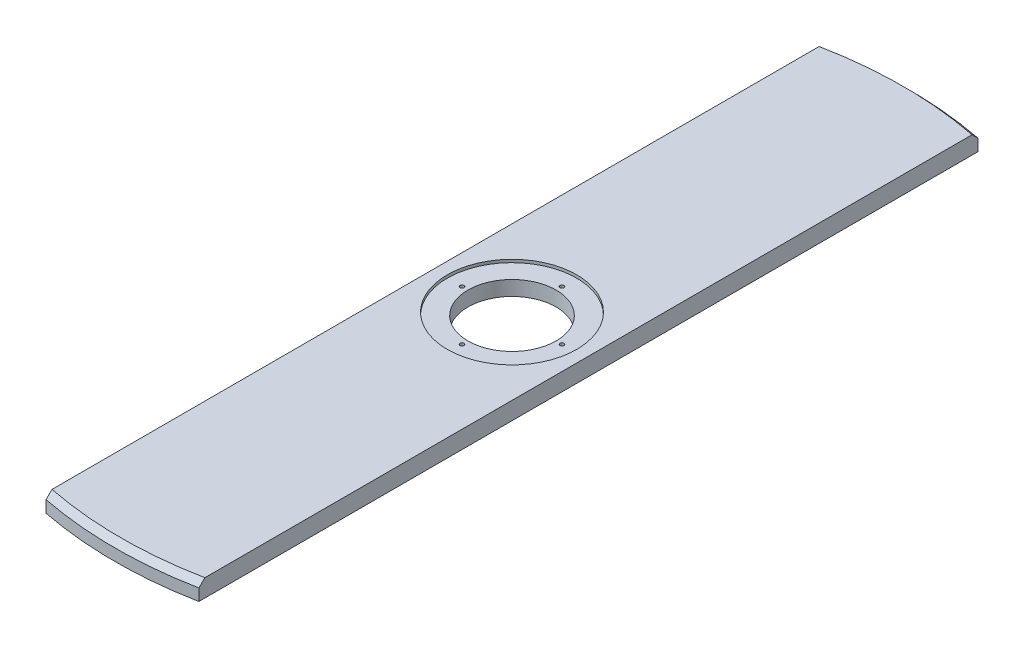
from build123d import *

# Parameters (mm, degrees)
SKETCH_1_R                = 810
EXTRUDE_1_DEPTH           = 25
SKETCH_2_R                = 730
EXTRUDE_2_DEPTH           = 5
CUT_EXTRUDE_1_REACH       = 1147.906
SKETCH_3_R                = 75
SKETCH_4_R                = 110
CUT_EXTRUDE_2_DEPTH       = 5
HOLE_WIZARD_M8_1_D        = 6.8
HOLE_WIZARD_25_5_25_5_1_D = 26
CUT_EXTRUDE_3_DEPTH       = 1146.905755287
CUT_EXTRUDE_3_DEPTH_BACK  = 1146.905755287
SKETCH_10_OUTSIDE_W       = 2080.244
SKETCH_10_OUTSIDE_H       = 2080.244
SKETCH_10_OUTSIDE_R       = 675
CHAMFER_1_SIZE            = 10


with BuildPart() as part:
    # 草图1 → 凸台-拉伸1 (new body)
    with BuildSketch(Plane(origin=(0, 0, 0), x_dir=(1, 0, 0), z_dir=(0, 1, 0))):
        with Locations(Location((0, 0, 0), (0, 0, 270))):
            Circle(SKETCH_1_R)
    extrude(amount=EXTRUDE_1_DEPTH)

    # 草图2 → 凸台-拉伸2 (add)
    with BuildSketch(Plane(origin=(0, 25, 0), x_dir=(1, 0, 0), z_dir=(0, 1, 0))):
        with Locations(Location((0, 0, 0), (0, 0, 270))):
            Circle(SKETCH_2_R)
    extrude(amount=EXTRUDE_2_DEPTH)

    # 草图3 → 切除-拉伸1 (cut, up to next)
    with BuildSketch(Plane(origin=(0, 30, 0), x_dir=(1, 0, 0), z_dir=(0, 1, 0)), mode=Mode.PRIVATE) as cut_extrude_1_sk1:
        with BuildLine():
            Line((130, 662.363193422), (130, -662.363193422))
            ThreePointArc((130, -662.363193422), (521.236510617, -428.879353665), (675, 0))
            ThreePointArc((675, 0), (521.236510617, 428.879353665), (130, 662.363193422))
        make_face()
    cut_extrude_1_tool1 = extrude(cut_extrude_1_sk1.sketch, amount=-CUT_EXTRUDE_1_REACH, mode=Mode.PRIVATE) & part.part
    # 草图3 → 切除-拉伸1 (cut, up to next)
    with BuildSketch(Plane(origin=(0, 30, 0), x_dir=(1, 0, 0), z_dir=(0, 1, 0)), mode=Mode.PRIVATE) as cut_extrude_1_sk2:
        with BuildLine():
            ThreePointArc((-130, 662.363193422), (-675, 0), (-130, -662.363193422))
            Line((-130, -662.363193422), (-130, 662.363193422))
        make_face()
    cut_extrude_1_tool2 = extrude(cut_extrude_1_sk2.sketch, amount=-CUT_EXTRUDE_1_REACH, mode=Mode.PRIVATE) & part.part
    # 草图3 → 切除-拉伸1 (cut, up to next)
    with BuildSketch(Plane(origin=(0, 30, 0), x_dir=(1, 0, 0), z_dir=(0, 1, 0)), mode=Mode.PRIVATE) as cut_extrude_1_sk3:
        with Locations(Location((0, 0, 0), (0, 0, 270))):
            Circle(SKETCH_3_R)
    cut_extrude_1_tool3 = extrude(cut_extrude_1_sk3.sketch, amount=-CUT_EXTRUDE_1_REACH, mode=Mode.PRIVATE) & part.part
    add(cut_extrude_1_tool1.solids().sort_by_distance((357.907844, 30, 0))[0], mode=Mode.SUBTRACT)
    add(cut_extrude_1_tool2.solids().sort_by_distance((-357.907844, 30, 0))[0], mode=Mode.SUBTRACT)
    add(cut_extrude_1_tool3.solids().sort_by_distance((0, 30, 0))[0], mode=Mode.SUBTRACT)

    # 草图4 → 切除-拉伸2 (cut)
    with BuildSketch(Plane(origin=(0, 30, 0), x_dir=(1, 0, 0), z_dir=(0, 1, 0))):
        with Locations(Location((0, 0, 0), (0, 0, 270))):
            Circle(SKETCH_4_R)
    extrude(amount=-CUT_EXTRUDE_2_DEPTH, mode=Mode.SUBTRACT)

    # M8 螺纹孔1 (through all)
    with Locations(Plane(origin=(0, 25, 0), x_dir=(1, 0, 0), z_dir=(0, 1, 0))):
        with Locations((0, 85), (85, 0), (0, -85), (-85, 0)):
            Hole(HOLE_WIZARD_M8_1_D / 2)

    # Ø25.5 (25.5) 直径孔1 (through all)
    with Locations(Plane(origin=(0, 25, 0), x_dir=(1, 0, 0), z_dir=(0, 1, 0))):
        with Locations((-59.354305918, 754.167962969), (59.354305918, 754.167962969), (176.601417757, 735.597844781), (289.500016584, 698.914866345), (395.270164208, 645.022284334), (491.307448562, 575.247112976), (575.247112976, 491.307448562), (645.022284334, 395.270164208), (698.914866345, 289.500016584), (735.597844781, 176.601417757), (754.167962969, 59.354305918), (754.167962969, -59.354305918), (735.597844781, -176.601417757), (698.914866345, -289.500016584), (645.022284334, -395.270164208), (575.247112976, -491.307448562), (491.307448562, -575.247112976), (395.270164208, -645.022284334), (289.500016584, -698.914866345), (176.601417757, -735.597844781), (59.354305918, -754.167962969), (-59.354305918, -754.167962969), (-176.601417757, -735.597844781), (-289.500016584, -698.914866345), (-395.270164208, -645.022284334), (-491.307448562, -575.247112976), (-575.247112976, -491.307448562), (-645.022284334, -395.270164208), (-698.914866345, -289.500016584), (-735.597844781, -176.601417757), (-754.167962969, -59.354305918), (-754.167962969, 59.354305918), (-735.597844781, 176.601417757), (-698.914866345, 289.500016584), (-645.022284334, 395.270164208), (-575.247112976, 491.307448562), (-491.307448562, 575.247112976), (-395.270164208, 645.022284334), (-289.500016584, 698.914866345), (-176.601417757, 735.597844781)):
            Hole(HOLE_WIZARD_25_5_25_5_1_D / 2)

    # 草图10 outside → 切除-拉伸3 (cut, two sides: drawn at the far end of the back side and taken through both)
    with BuildSketch(Plane(origin=(0, 30, 0), x_dir=(1, 0, 0), z_dir=(0, 1, 0)).offset(-CUT_EXTRUDE_3_DEPTH_BACK)):
        Rectangle(SKETCH_10_OUTSIDE_W, SKETCH_10_OUTSIDE_H)
        Circle(SKETCH_10_OUTSIDE_R, mode=Mode.SUBTRACT)
    extrude(amount=CUT_EXTRUDE_3_DEPTH + CUT_EXTRUDE_3_DEPTH_BACK, mode=Mode.SUBTRACT)

    # 倒角1
    chamfer_1_edges = [part.edges().sort_by_distance(p)[0] for p in [
        (0, 30, -675),
        (0, 30, 675),
    ]]
    chamfer(chamfer_1_edges, length=CHAMFER_1_SIZE)


solid = part.part
